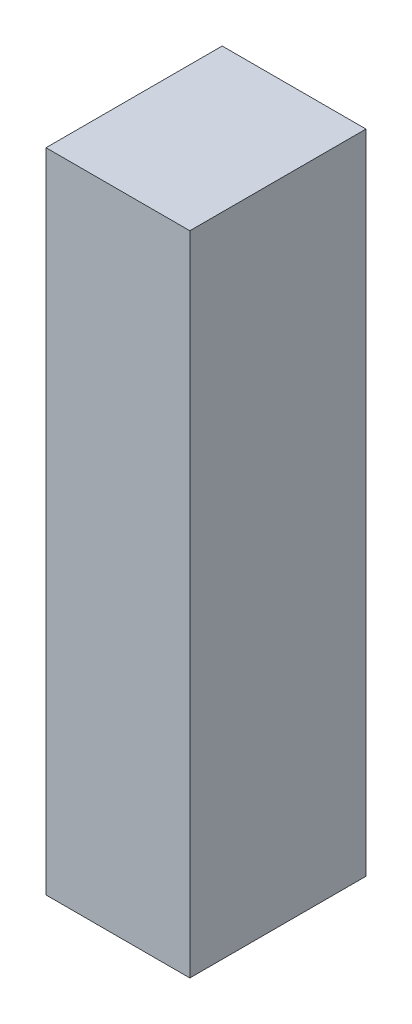
SolidWorks part; units mm, degrees
ref_plane "前视基准面" through (0, 0, 0) normal (0, 0, 1) x (1, 0, 0)
ref_plane "上视基准面" through (0, 0, 0) normal (0, 1, 0) x (1, 0, 0)
ref_plane "右视基准面" through (0, 0, 0) normal (1, 0, 0) x (0, 0, -1)
sketch "草图1" plane through (0, 0, 0) normal (0, 0, 1) x (1, 0, 0)
  line L1 (0, 45) -> (20, 45)
  line L2 (0, 45) -> (0, -45)
  line L3 (0, -45) -> (20, -45)
  line L4 (20, 45) -> (20, -45)
  dimension "D1" = 90
  dimension "D2" = 20
extrude "凸台-拉伸1" add sketch "草图1" along normal blind 24.5
